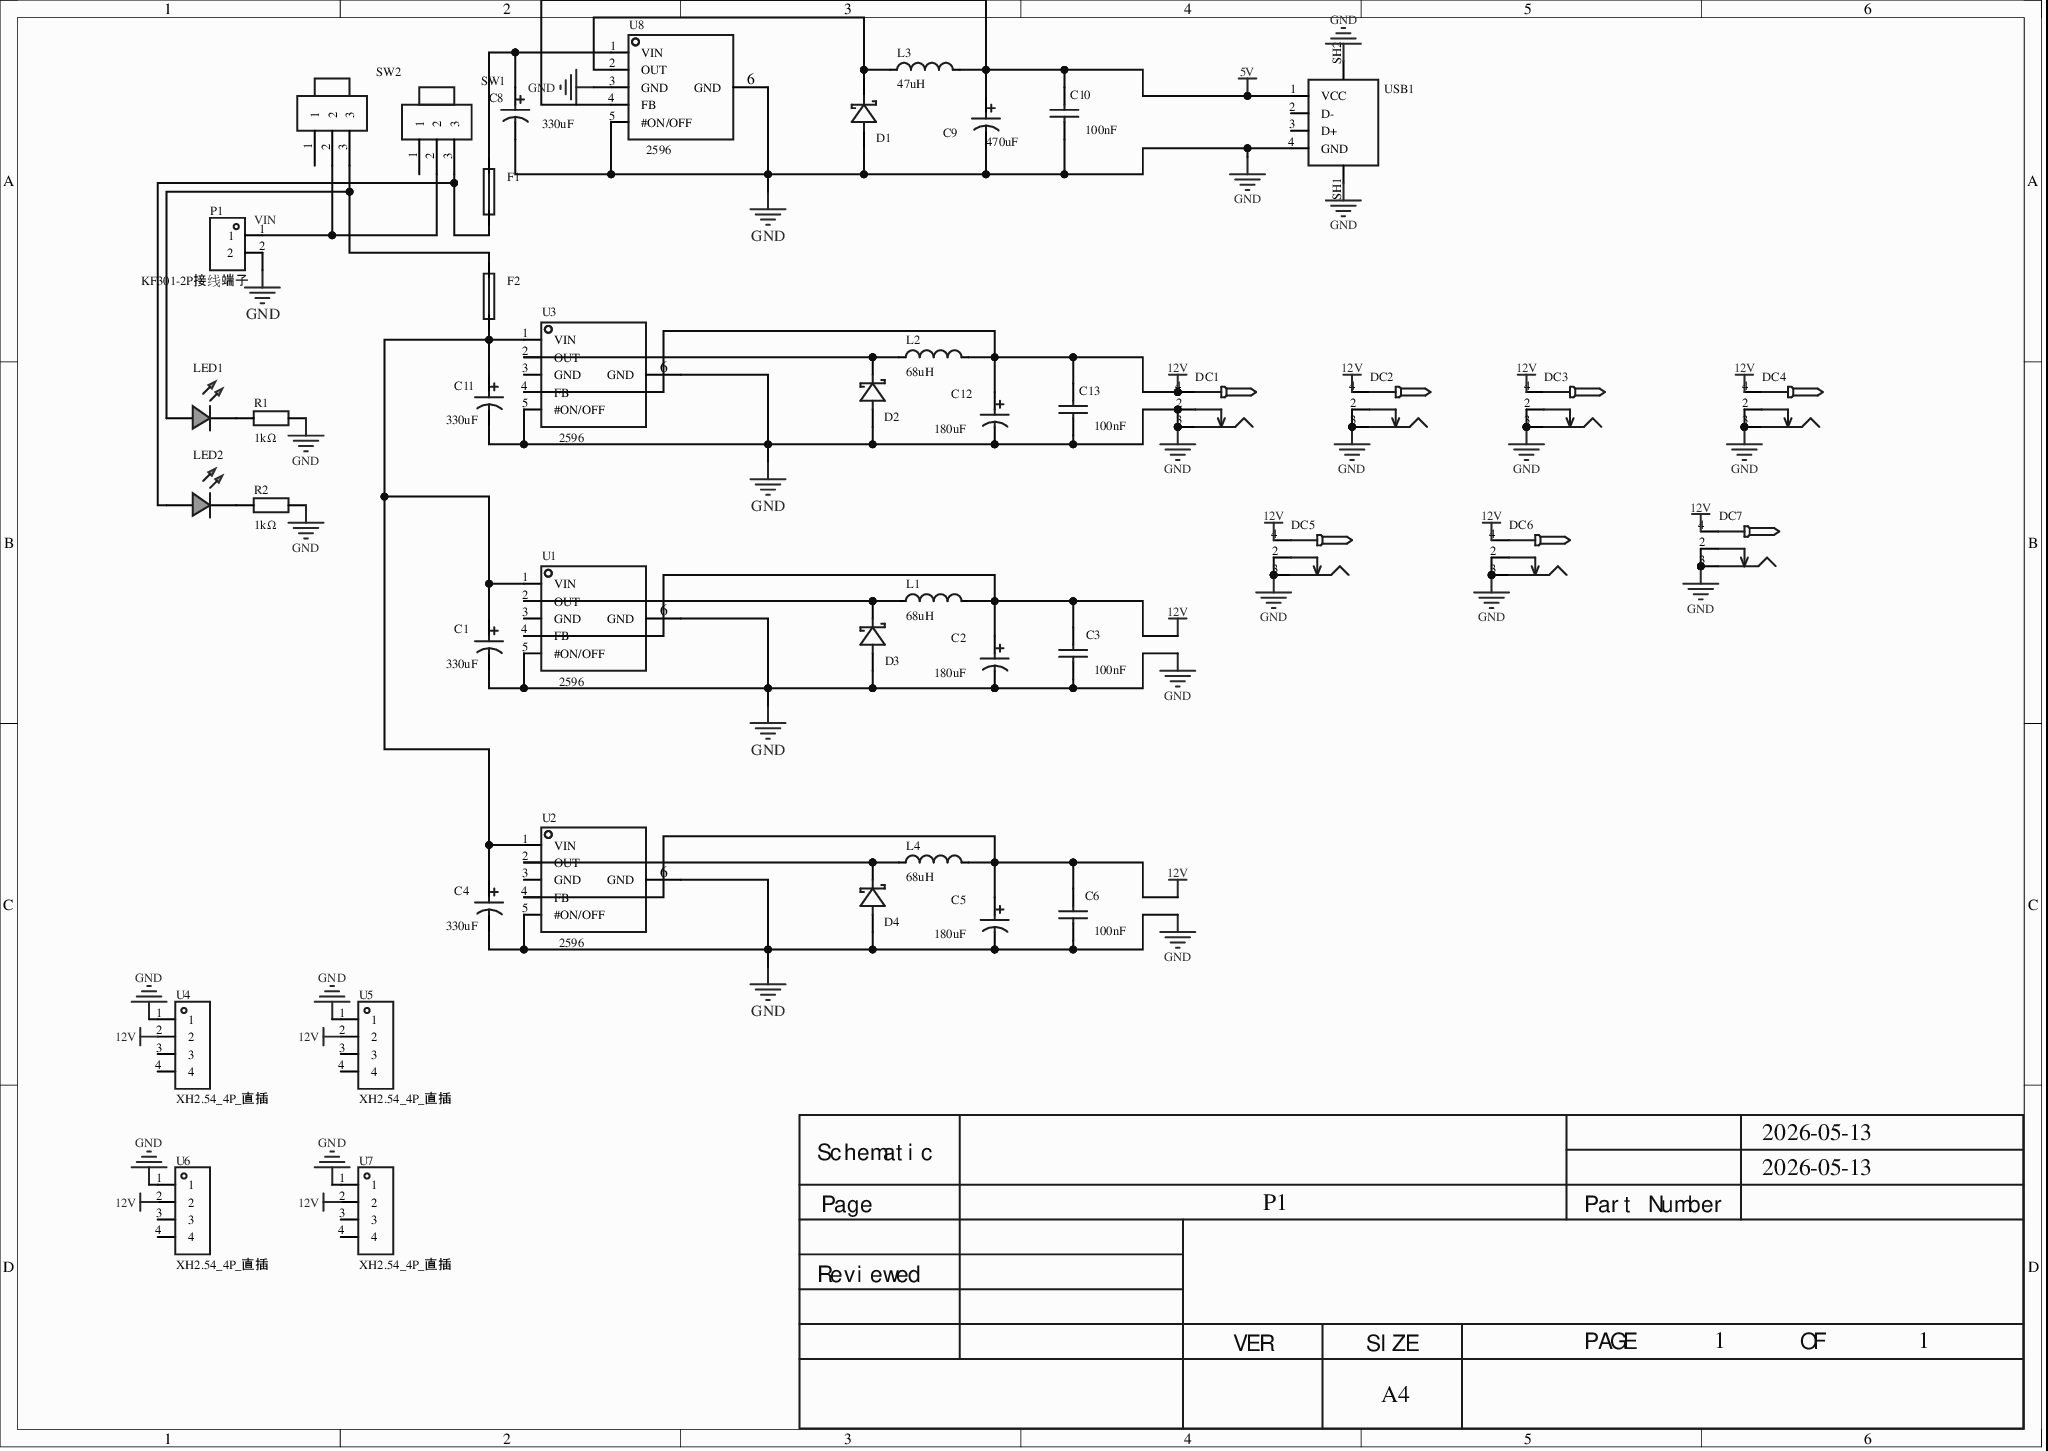
[diagram p0: MISC49942-3.schdoc]
# Altium project MISC49942-2.PrjPcb
1 sheet, 45 parts. Net scope: global (net labels, ports and power ports of the same name join across sheets).
Board file: MISC49942.pcbdoc

## Sheet MISC49942-3.schdoc
size 297 x 210 mm; Version: V1.0; @Project Name: MISC49942; @Page Count: 1; @Update Date: 2026-05-13; @Create Date: 2026-05-13; @Schematic Name: MISC49942; @Page No: 1

### Parts
C1  value 330uF  [CAP-SMD_BD8.0-L8.3-W8.3-RD]
C2  value 180uF  [CAP-SMD_BD8.0-L8.3-W8.3-RD]
C3  value 100nF  [C0805]
C4  value 330uF  [CAP-SMD_BD8.0-L8.3-W8.3-RD]
C5  value 180uF  [CAP-SMD_BD8.0-L8.3-W8.3-RD]
C6  value 100nF  [C0805]
C8  value 330uF  [CAP-SMD_BD8.0-L8.3-W8.3-RD]
C9  value 470uF  [CAP-SMD_BD8.0-L8.3-W8.3-RD]
C10  value 100nF  [C0805]
C11  value 330uF  [CAP-SMD_BD8.0-L8.3-W8.3-RD]
C12  value 180uF  [CAP-SMD_BD8.0-L8.3-W8.3-RD]
C13  value 100nF  [C0805]
D1  (no value)  [SMA_L4.3-W2.6-LS5.2-RD]
D2  (no value)  [SMA_L4.3-W2.6-LS5.2-RD]
D3  (no value)  [SMA_L4.3-W2.6-LS5.2-RD]
D4  (no value)  [SMA_L4.3-W2.6-LS5.2-RD]
DC1  (no value)  [DC-2.0]
DC2  (no value)  [DC-2.0]
DC3  (no value)  [DC-2.0]
DC4  (no value)  [DC-2.0]
DC5  (no value)  [DC-2.0]
DC6  (no value)  [DC-2.0]
DC7  (no value)  [DC-2.0]
F1  10A保险丝  [FUSE-SMD_L6.1-W2.6]  (value not drawn)
F2  10A保险丝  [FUSE-SMD_L6.1-W2.6]  (value not drawn)
L1  value 68uH  [IND-SMD_L7.0-W6.6]
L2  value 68uH  [IND-SMD_L7.0-W6.6]
L3  value 47uH  [IND-SMD_L7.0-W6.6]
L4  value 68uH  [IND-SMD_L7.0-W6.6]
LED1  (no value)  [LED_TH-3mm]
LED2  (no value)  [LED_TH-3mm]
P1  KF301-2P接线端子  [CONN-TH_XY301V-A-5.0-2P]
R1  1kΩ  [Res_1/8W]
R2  1kΩ  [Res_1/8W]
SW1  船型开关601-10211BB  [SW-TH_601-10211BB]  (value not drawn)
SW2  船型开关601-10211BB  [SW-TH_601-10211BB]  (value not drawn)
U1  LM2596S-12  [TO-263-5_L10.0-W8.4-P1.70-LS15.3-BR]  (value not drawn)
U2  LM2596S-12  [TO-263-5_L10.0-W8.4-P1.70-LS15.3-BR]  (value not drawn)
U3  LM2596S-12  [TO-263-5_L10.0-W8.4-P1.70-LS15.3-BR]  (value not drawn)
U4  XH2.54_4P_直插  [CONN-TH_4P-P2.50-XH2.54-4P]
U5  XH2.54_4P_直插  [CONN-TH_4P-P2.50-XH2.54-4P]
U6  XH2.54_4P_直插  [CONN-TH_4P-P2.50-XH2.54-4P]
U7  XH2.54_4P_直插  [CONN-TH_4P-P2.50-XH2.54-4P]
U8  LM2596S-5.0  [TO-263-5_L10.2-W8.9-P1.70-BR]  (value not drawn)
USB1  (no value)  [USB_ Type-A]

### Nets
5V: C9.1 C10.1 L3.2 U8.4(FB) USB1.1(VCC)
12V: C2.1 C3.1 C5.1 C6.1 C12.1 C13.1 DC1.4 DC2.4 DC3.4 DC4.4 DC5.4 DC6.4 DC7.4 L1.2 L2.2 L4.2 U1.4(FB) U2.4(FB) U3.4(FB) U4.2 U5.2 U6.2 U7.2
GND: C1.2 C2.2 C3.2 C4.2 C5.2 C6.2 C8.2 C9.2 C10.2 C11.2 C12.2 C13.2 D1.2(A) D2.2(A) D3.2(A) D4.2(A) DC1.2 DC1.3 DC2.2 DC2.3 DC3.2 DC3.3 DC4.2 DC4.3 DC5.2 DC5.3 DC6.2 DC6.3 DC7.2 DC7.3 P1.2 R1.2 R2.2 U1.5(#ON/OFF) U1.6(GND) U2.5(#ON/OFF) U2.6(GND) U3.5(#ON/OFF) U3.6(GND) U4.1 U5.1 U6.1 U7.1 U8.3(GND) U8.5(#ON/OFF) U8.6(GND) USB1.4(GND) USB1.SH1 USB1.SH2
NetC1_1: C1.1 C4.1 C11.1 F2.1 U1.1(VIN) U2.1(VIN) U3.1(VIN)
NetC8_1: C8.1 F1.2 U8.1(VIN)
NetD1_1: D1.1(K) L3.1 U8.2(OUT)
NetD2_1: D2.1(K) L2.1 U3.2(OUT)
NetD3_1: D3.1(K) L1.1 U1.2(OUT)
NetD4_1: D4.1(K) L4.1 U2.2(OUT)
NetF1_1: F1.1 LED2.1(C) SW1.3
NetF2_2: F2.2 LED1.1(C) SW2.3
NetLED1_2: LED1.2(A) R1.1
NetLED2_2: LED2.2(A) R2.1
NetP1_1: P1.1 SW1.2 SW2.2

Not connected (* = marked no-connect by the designer): SW1 1; SW2 1; U1 3(GND); U2 3(GND); U3 3(GND); U4 3 4; U5 3 4; U6 3 4; U7 3 4; USB1 2(D-) 3(D+)

### Notes on the sheet
- Labels drawn without touching a wire or pin: VIN
- 2026-05-13
- Schematic
- Page
- P1
- Part Number
- Reviewed
- VER
- SIZE
- A4
- PAGE
- 1
- OF

### Library data of the parts
C1 C2 C4 C5 = CS1V221M-CRF10　: 容值:220uF;精度:±20%;额定电压:35V;电容体直径:8mm;电容体长度:10.5mm;纹波电流:-;等效串联电阻:-;工作寿命:2000hrs@105;工作温度:-40~+105;; Manufacturer: ST(先科); Rated Voltage: 25V; 3D Model: b102f1362be24624a1b1334fec8dc7f4; 3D Model Transform: 354.33,326.81037,0,0,0,0,0,0,0; Tolerance: ±20%; φD: 8mm; L: 10.5mm; AddInBom: yes; Symbol: CS1V221M-CRF10; Device: CS1V221M-CRF10; Lifetime @ Temp: 2000hrs@105; Operating Temperature: -40~+105; Manufacturer Part: CS1V221M-CRF10; Supplier Footprint: SMD,8x10.5mm; JLCPCB Part Class: Extended Part; Datasheet: https://atta.szlcsc.com/upload/public/pdf/source/20170325/1490427945143.pdf; Supplier: LCSC; Ripple Current: -; Equivalent Series Resistance(ESR): -; ConvertToPcb: yes; FootprintName: CAP-SMD_BD8.0-L8.3-W8.3-RD; ModelName: CAP-SMD_BD8.0-L8.3-W8.3-RD
  C1 C4: Supplier Part: C97814
C3 C6 = CL21B104KBCNNNC: 容值:100nF;精度:±10%;额定电压:50V;温度系数:X7R;; Manufacturer: SAMSUNG(三星); 3D Model: 1ba041120af144c991958decab20d241; 3D Model Transform: 78.74,51.181,0,0,0,0,0,0.0005,0; Tolerance: ±10%; Voltage Rated: 50V; Temperature Coefficient: X7R; AddInBom: yes; ModelName: C0805_L2.0-W1.3-H1.3; Symbol: CL21B104KBCNNNC; Device: CL21B104KBCNNNC; LCSC Part Name: 100nF ±10% 50V; Supplier Part: C1711; Manufacturer Part: CL21B104KBCNNNC; Supplier Footprint: 0805; JLCPCB Part Class: Extended Part; Datasheet: https://atta.szlcsc.com/upload/public/pdf/source/20160103/1457707693305.pdf; Supplier: LCSC; ConvertToPcb: yes; FootprintName: C0805
C8 C9 C11 C12 = CS1V221M-CRF10　: 容值:220uF;精度:±20%;额定电压:35V;电容体直径:8mm;电容体长度:10.5mm;纹波电流:-;等效串联电阻:-;工作寿命:2000hrs@105;工作温度:-40~+105;; Manufacturer: ST(先科); Rated Voltage: 25V; AddInBom: yes; ModelId: b102f1362be24624a1b1334fec8dc7f4; ModelTransform: 354.33,326.81037,0,0,0,0,0,0,0; Tolerance: ±20%; φD: 8mm; L: 10.5mm; Lifetime @ Temp: 2000hrs@105; Operating Temperature: -40~+105; Device: CS1V221M-CRF10; Symbol: CS1V221M-CRF10; ManufacturerPart: CS1V221M-CRF10; Supplier Footprint: SMD,8x10.5mm; JLCPCB Part Class: Extended Part; Datasheet: https://atta.szlcsc.com/upload/public/pdf/source/20170325/1490427945143.pdf; Supplier: LCSC; ConvertToPcb: yes; FootprintName: CAP-SMD_BD8.0-L8.3-W8.3-RD; ModelName: CAP-SMD_BD8.0-L8.3-W8.3-RD; Ripple Current: -; Equivalent Series Resistance(ESR): -
  C8 C11: SupplierPart: C97814
C10 C13 = CL21B104KBCNNNC: 容值:100nF;精度:±10%;额定电压:50V;温度系数:X7R;; Manufacturer: SAMSUNG(三星); AddInBom: yes; ModelId: 1ba041120af144c991958decab20d241; ModelName: C0805_L2.0-W1.3-H1.3; ModelTransform: 78.74,51.181,0,0,0,0,0,0.0005,0; Tolerance: ±10%; Voltage Rated: 50V; Temperature Coefficient: X7R; Device: CL21B104KBCNNNC; Symbol: CL21B104KBCNNNC; LCSC Part Name: 100nF ±10% 50V; SupplierPart: C1711; ManufacturerPart: CL21B104KBCNNNC; Supplier Footprint: 0805; JLCPCB Part Class: Extended Part; Datasheet: https://atta.szlcsc.com/upload/public/pdf/source/20160103/1457707693305.pdf; Supplier: LCSC; ConvertToPcb: yes; FootprintName: C0805
D1 D2 = SS34_3: Manufacturer: TDD(台冠电子); ManufacturerPart: SS34; Symbol: SS34_C3032484; AddInBom: yes; ModelId: 7ed2c9d0a4a74bbdbba07ab4052caf5b; ModelTransform: 185.039,102.362,0,0,0,0,0,0,0; Device: SS34_3; LCSC Part Name: SS34; SupplierPart: C3032484; Supplier Footprint: SMA; JLCPCB Part Class: Extended Part; Datasheet: https://atta.szlcsc.com/upload/public/pdf/source/20220622/9D70D0693761B542BF6F533590093AA5.pdf; Supplier: LCSC; ConvertToPcb: yes; FootprintName: SMA_L4.3-W2.6-LS5.2-RD; ModelName: SMA_L4.3-W2.6-LS5.2-RD
D3 D4 = SS34_3: Manufacturer: TDD(台冠电子); Manufacturer Part: SS34; Symbol: SS34_C3032484; 3D Model: 7ed2c9d0a4a74bbdbba07ab4052caf5b; 3D Model Transform: 185.039,102.362,0,0,0,0,0,0,0; AddInBom: yes; Device: SS34_3; LCSC Part Name: SS34; Supplier Part: C3032484; Supplier Footprint: SMA; JLCPCB Part Class: Extended Part; Datasheet: https://atta.szlcsc.com/upload/public/pdf/source/20220622/9D70D0693761B542BF6F533590093AA5.pdf; Supplier: LCSC; ConvertToPcb: yes; FootprintName: SMA_L4.3-W2.6-LS5.2-RD; ModelName: SMA_L4.3-W2.6-LS5.2-RD
DC1-DC7 = DC-005_2.0: Symbol: DC电源接口; ConvertToPcb: yes; ModelId: f5f20b8a2308479b936ba3c2698865bb0819f05c4eef4c71ace90d822a990e87; ModelName: DC-IN-TH_DC-5520-1; ModelTransform: 372.05,551.18,582.68,90,0,0,137.8,0,-149.61; Device: DC-005_2.0; AddInBom: yes; Supplier Footprint: 插件; FootprintName: DC-2.0
F1 F2 = 10A保险丝: AddInBom: yes; ModelId: 8dc97aad3e5d43c2b990fd56287574220819f05c4eef4c71ace90d822a990e87; ModelName: FUSE-SMD_L6.1-W2.6-H2.6; ModelTransform: 240.157,102.362,0,0,0,0,0,0,0; Symbol: 10A保险丝; Device: 10A保险丝; LCSC Part Name: 10A保险丝; SupplierPart: C9900011494; ManufacturerPart: 10A保险丝; Supplier Footprint: 1808; JLCPCB Part Class: Extended Part; Supplier: LCSC; ConvertToPcb: yes; FootprintName: FUSE-SMD_L6.1-W2.6
L1 L4 = CMLO0630H330MTT: 电感值:33uH;精度:±20%;直流电阻(DCR):270mΩ;; Manufacturer: Cybermax(思博科技); 3D Model: 6860c29aec394a38a0f014af7f722a42; 3D Model Transform: 275.6,259.8,0,0,0,0,0,0,0; Tolerance: ±20%; DC Resistance (DCR): 270mΩ; AddInBom: yes; ModelName: IND-SMD_L7.0-W6.6-H3.0; Symbol: CMLO0630H330MTT; Device: CMLO0630H330MTT; LCSC Part Name: 33uH ±20% 270mΩ; Manufacturer Part: CMLO0630H330MTT; Supplier Footprint: SMD; JLCPCB Part Class: Extended Part; Datasheet: https://atta.szlcsc.com/upload/public/pdf/source/20201124/C961478_55C23F293F63DC1D2CF3D7AB16D0E182.pdf; Supplier: LCSC; ConvertToPcb: yes; FootprintName: IND-SMD_L7.0-W6.6
L2 L3 = CMLO0630H330MTT: 电感值:33uH;精度:±20%;直流电阻(DCR):270mΩ;; Manufacturer: Cybermax(思博科技); AddInBom: yes; ModelId: 6860c29aec394a38a0f014af7f722a42; ModelName: IND-SMD_L7.0-W6.6-H3.0; ModelTransform: 275.6,259.8,0,0,0,0,0,0,0; Tolerance: ±20%; DC Resistance (DCR): 270mΩ; Device: CMLO0630H330MTT; Symbol: CMLO0630H330MTT; LCSC Part Name: 33uH ±20% 270mΩ; ManufacturerPart: CMLO0630H330MTT; Supplier Footprint: SMD; JLCPCB Part Class: Extended Part; Datasheet: https://atta.szlcsc.com/upload/public/pdf/source/20201124/C961478_55C23F293F63DC1D2CF3D7AB16D0E182.pdf; Supplier: LCSC; ConvertToPcb: yes; FootprintName: IND-SMD_L7.0-W6.6
LED1 LED2 = LED_TH-G_3mm: AddInBom: yes; ModelId: 07c881668c9448ef9b36eb6a2126ca130819f05c4eef4c71ace90d822a990e87; ModelName: LED-TH-3mm_G; ModelTransform: 141.27444,153.32669525336098,354.32999763315956,0,0,0,-5.90551,0,-137.79528; Symbol: LED_TH-G; Device: LED_TH-G_3mm; ConvertToPcb: yes; FootprintName: LED_TH-3mm; Supplier Footprint: 插件
P1 = KF301-2P接线端子: AddInBom: yes; ModelId: ef7ead88b0f2448d904975b26718870f0819f05c4eef4c71ace90d822a990e87; ModelTransform: 417.322,299.212,0,0,0,0,11.811,-7.835,-157.48; Symbol: KF301-2P接线端子; Device: KF301-2P接线端子; LCSC Part Name: KF301-2P接线端子; SupplierPart: C9900016950; ManufacturerPart: KF301-2P接线端子; Supplier Footprint: CK301-2P; JLCPCB Part Class: Extended Part; Supplier: LCSC; ConvertToPcb: yes; FootprintName: CONN-TH_XY301V-A-5.0-2P; ModelName: CONN-TH_XY301V-A-5.0-2P
R1 R2 = Res_AXIAL-1/8W: Symbol: 电阻; ConvertToPcb: yes; ModelId: b2b5ae7ae4c642178fe0039925c86a3f; ModelName: RES-TH_BD1.8-L3.2-P7.20-D0.4; ModelTransform: 282.86,66.88,253.09,0,0,0,0,0,-191; Device: Res_AXIAL-1/8W; Value: 1kΩ; AddInBom: yes; Supplier Footprint: 轴向引线; FootprintName: Res_1/8W
SW1 SW2 = 船型开关601-10211BB: Symbol: Rocker switch601-10211BB; AddInBom: yes; ModelId: 84d8922f25fd40a6bb3cbb8778d0ac1f0819f05c4eef4c71ace90d822a990e87; ModelTransform: 830.707,594.487,0,0,0,0,0,0,-196.85; Device: 船型开关601-10211BB; LCSC Part Name: 船型开关601-10211BB; SupplierPart: C67849; ManufacturerPart: 船型开关601-10211BB; Supplier Footprint: 直脚 三脚两档; JLCPCB Part Class: Extended Part; Supplier: LCSC; ConvertToPcb: yes; FootprintName: SW-TH_601-10211BB; ModelName: SW-TH_601-10211BB
U1 U2 = LM2596S-12_C347422: Manufacturer: UMW(广东友台半导体); Symbol: LM2596-TO263; Add into BOM: yes; 3D Model: fb036f748a274327bb376552b66e43ac; 3D Model Transform: 388.9756,661.416,0,90,0,0,-43.311,0,0; Device: LM2596S-12_C347422; Convert to PCB: yes; LCSC Part Name: DC-DC芯片; Supplier Part: C347422; Manufacturer Part: LM2596S-12; Supplier Footprint: TO-263; JLCPCB Part Class: Extended Part; Datasheet: https://atta.szlcsc.com/upload/public/pdf/source/20211011/C7416AEF3194BD283261B8F2553C4145.pdf; Supplier: LCSC; FootprintName: TO-263-5_L10.0-W8.4-P1.70-LS15.3-BR; ModelName: TO-263-5_L10.0-W8.4-P1.70-LS15.3-BR
U3 = LM2596S-12_C347422: Manufacturer: UMW(广东友台半导体); Symbol: LM2596-TO263; Add into BOM: yes; ModelId: fb036f748a274327bb376552b66e43ac; ModelTransform: 388.9756,661.416,0,90,0,0,-43.311,0,0; Convert to PCB: yes; Device: LM2596S-12_C347422; LCSC Part Name: DC-DC芯片; SupplierPart: C347422; ManufacturerPart: LM2596S-12; Supplier Footprint: TO-263; JLCPCB Part Class: Extended Part; Datasheet: https://atta.szlcsc.com/upload/public/pdf/source/20211011/C7416AEF3194BD283261B8F2553C4145.pdf; Supplier: LCSC; FootprintName: TO-263-5_L10.0-W8.4-P1.70-LS15.3-BR; ModelName: TO-263-5_L10.0-W8.4-P1.70-LS15.3-BR
U4-U7 = XH2.54_4P_直插: AddInBom: yes; ModelId: c69236e4c0a047c6aeeeefc1552045f50819f05c4eef4c71ace90d822a990e87; ModelTransform: 492.125,228.346,0,180,0,0,0,-19.685,-137.795; Symbol: XH2.54_4P_直插; Device: XH2.54_4P_直插; LCSC Part Name: XH2.54_4P_直插; SupplierPart: C9900008616; ManufacturerPart: XH2.54_4P_直插; Supplier Footprint: XH2.54_4P; JLCPCB Part Class: Extended Part; Supplier: LCSC; ConvertToPcb: yes; FootprintName: CONN-TH_4P-P2.50-XH2.54-4P; ModelName: CONN-TH_4P-P2.50-XH2.54-4P
U8 = LM2596S-5.0_C347421: 功能类型:降压型;输出类型:固定;输入电压:40V;输出电压:5V;输出电流(最大值):3A;; Manufacturer: UMW(广东友台半导体); Symbol: LM2596-TO263; Add into BOM: yes; 3D Model: 4e421a816a7f4d57b8710832ddea550a; 3D Model Transform: 401.574,560.17797,0,90,0,0,-45.276,0,0; Function: 降压型; Synchronous Rectification: 否; Output Type: 固定; Number of Outputs: 1; Topology: 降压式; Input Voltage: 40V; Output Voltage: 5V; Output Current (Max): 3A; Switching Frequency: 150kHz; ModelName: TO-263-5-5P_L10.2-W8.7-H4.5-LS14.4-P1.70; Convert to PCB: yes; Device: LM2596S-5.0_C347421; LCSC Part Name: 降压型 输入40V 输出5V 3A; Supplier Part: C347421; Manufacturer Part: LM2596S-5.0; Supplier Footprint: TO-263-5; JLCPCB Part Class: Extended Part; Datasheet: https://atta.szlcsc.com/upload/public/pdf/source/20211011/C7416AEF3194BD283261B8F2553C4145.pdf; Supplier: LCSC; Operating Temperature: -40℃~+125℃@(TA); FootprintName: TO-263-5_L10.2-W8.9-P1.70-BR
USB1 = USB_ Type-A: AddInBom: yes; ModelId: 0a0bfc60af8549fa93b7465d8aaf02b10819f05c4eef4c71ace90d822a990e87; ModelName: USB-A-TH__USB-AF-90; ModelTransform: 612.05,551.18,446.85,0,0,0,0,-15.75,-157.48; Symbol: USB_Type-A; Device: USB_ Type-A; ConvertToPcb: yes; FootprintName: USB_ Type-A; Supplier Footprint: 插件